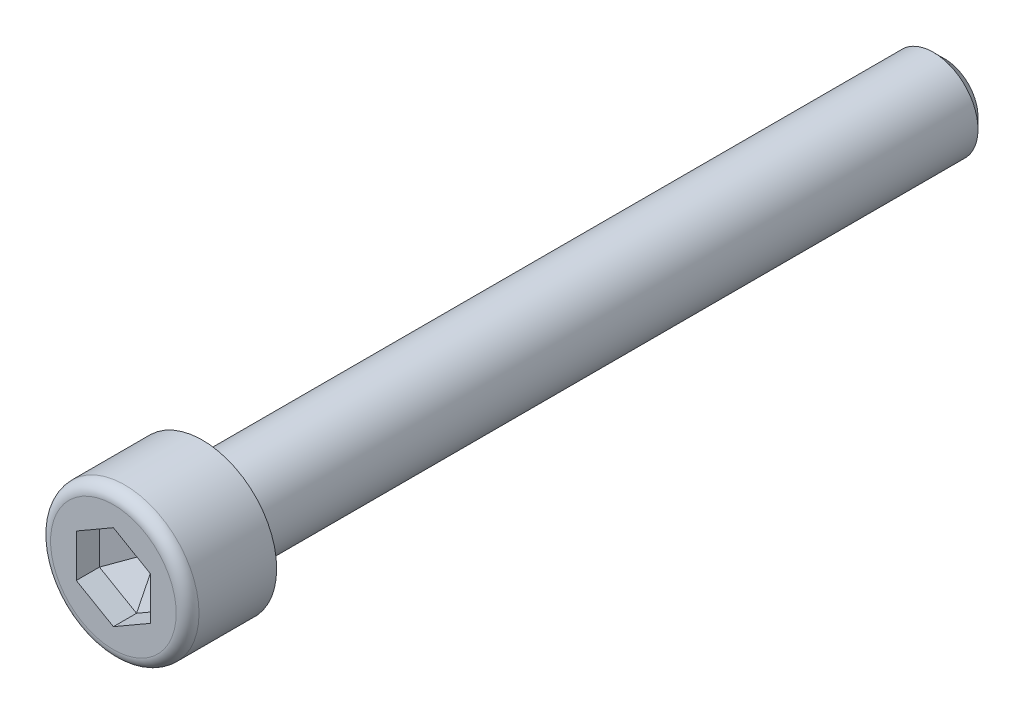
from build123d import *
from OCP.BRepFilletAPI import BRepFilletAPI_MakeChamfer

# Parameters (mm, degrees)
SKETCH1_R           = 5
BOSS_EXTRUDE1_DEPTH = 6
CUT_EXTRUDE1_DEPTH  = 3
SKETCH3_R           = 3
BOSS_EXTRUDE2_DEPTH = 50
CHAMFER1_SIZE       = 0.75
FILLET1_R           = 0.769230769
CHAMFER2_SIZE       = 1.44092219
CHAMFER2_SIZE2      = 2.495750443
FILLET2_R           = 0.1


with BuildPart() as part:
    # Sketch1 → Boss-Extrude1 (new body)
    with BuildSketch(Plane.XY):
        Circle(SKETCH1_R)
    extrude(amount=BOSS_EXTRUDE1_DEPTH)

    # Sketch2 → Cut-Extrude1 (cut)
    with BuildSketch(Plane.XY.offset(6)):
        Polygon((2.5, 1.443375673), (0, 2.886751346), (-2.5, 1.443375673), (-2.5, -1.443375673), (0, -2.886751346), (2.5, -1.443375673), align=None)
    extrude(amount=-CUT_EXTRUDE1_DEPTH, mode=Mode.SUBTRACT)

    # Sketch3 → Boss-Extrude2 (add)
    with BuildSketch(Plane(origin=(0, 0, 0), x_dir=(-1, 0, 0), z_dir=(0, 0, -1))):
        with Locations(Location((0, 0, 0), (0, 0, 180))):
            Circle(SKETCH3_R)
    extrude(amount=BOSS_EXTRUDE2_DEPTH)

    # Chamfer1
    chamfer1_edges = [part.edges().sort_by_distance(p)[0] for p in [
        (-3, 0, -50),
    ]]
    chamfer(chamfer1_edges, length=CHAMFER1_SIZE)

    # Fillet1
    fillet1_edges = [part.edges().sort_by_distance(p)[0] for p in [
        (-5, 0, 6),
    ]]
    fillet(fillet1_edges, radius=FILLET1_R)

    # Chamfer2: one chamfer whose edges measure the first distance from different faces: ONE call of the kernel's chamfer builder (chamfer() names one face for all edges)
    chamfer2_edges_1 = [part.edges().sort_by_distance(p)[0] for p in [
        (-1.25, 2.165063509, 3),
    ]]
    chamfer2_side_1 = [part.faces().sort_by_distance(p)[0] for p in [
        (-1.25, 2.165063509, 4.5),
    ]]
    chamfer2_edges_2 = [part.edges().sort_by_distance(p)[0] for p in [
        (1.25, 2.165063509, 3),
    ]]
    chamfer2_side_2 = [part.faces().sort_by_distance(p)[0] for p in [
        (1.25, 2.165063509, 4.5),
    ]]
    chamfer2_edges_3 = [part.edges().sort_by_distance(p)[0] for p in [
        (2.5, 0, 3),
    ]]
    chamfer2_side_3 = [part.faces().sort_by_distance(p)[0] for p in [
        (2.5, 0, 4.5),
    ]]
    chamfer2_edges_4 = [part.edges().sort_by_distance(p)[0] for p in [
        (1.25, -2.165063509, 3),
    ]]
    chamfer2_side_4 = [part.faces().sort_by_distance(p)[0] for p in [
        (1.25, -2.165063509, 4.5),
    ]]
    chamfer2_edges_5 = [part.edges().sort_by_distance(p)[0] for p in [
        (-1.25, -2.165063509, 3),
    ]]
    chamfer2_side_5 = [part.faces().sort_by_distance(p)[0] for p in [
        (-1.25, -2.165063509, 4.5),
    ]]
    chamfer2_edges_6 = [part.edges().sort_by_distance(p)[0] for p in [
        (-2.5, 0, 3),
    ]]
    chamfer2_side_6 = [part.faces().sort_by_distance(p)[0] for p in [
        (-2.5, 0, 4.5),
    ]]
    chamfer2 = BRepFilletAPI_MakeChamfer(part.part.solid().wrapped)
    for e in chamfer2_edges_1:
        chamfer2.Add(CHAMFER2_SIZE, CHAMFER2_SIZE2, e.wrapped, chamfer2_side_1[0].wrapped)  # the first distance lies on this face
    for e in chamfer2_edges_2:
        chamfer2.Add(CHAMFER2_SIZE, CHAMFER2_SIZE2, e.wrapped, chamfer2_side_2[0].wrapped)  # the first distance lies on this face
    for e in chamfer2_edges_3:
        chamfer2.Add(CHAMFER2_SIZE, CHAMFER2_SIZE2, e.wrapped, chamfer2_side_3[0].wrapped)  # the first distance lies on this face
    for e in chamfer2_edges_4:
        chamfer2.Add(CHAMFER2_SIZE, CHAMFER2_SIZE2, e.wrapped, chamfer2_side_4[0].wrapped)  # the first distance lies on this face
    for e in chamfer2_edges_5:
        chamfer2.Add(CHAMFER2_SIZE, CHAMFER2_SIZE2, e.wrapped, chamfer2_side_5[0].wrapped)  # the first distance lies on this face
    for e in chamfer2_edges_6:
        chamfer2.Add(CHAMFER2_SIZE, CHAMFER2_SIZE2, e.wrapped, chamfer2_side_6[0].wrapped)  # the first distance lies on this face
    add(Compound.cast(chamfer2.Shape()), mode=Mode.REPLACE)

    # Fillet2
    fillet2_edges = [part.edges().sort_by_distance(p)[0] for p in [
        (-3, 0, 0),
    ]]
    fillet(fillet2_edges, radius=FILLET2_R)


solid = part.part
